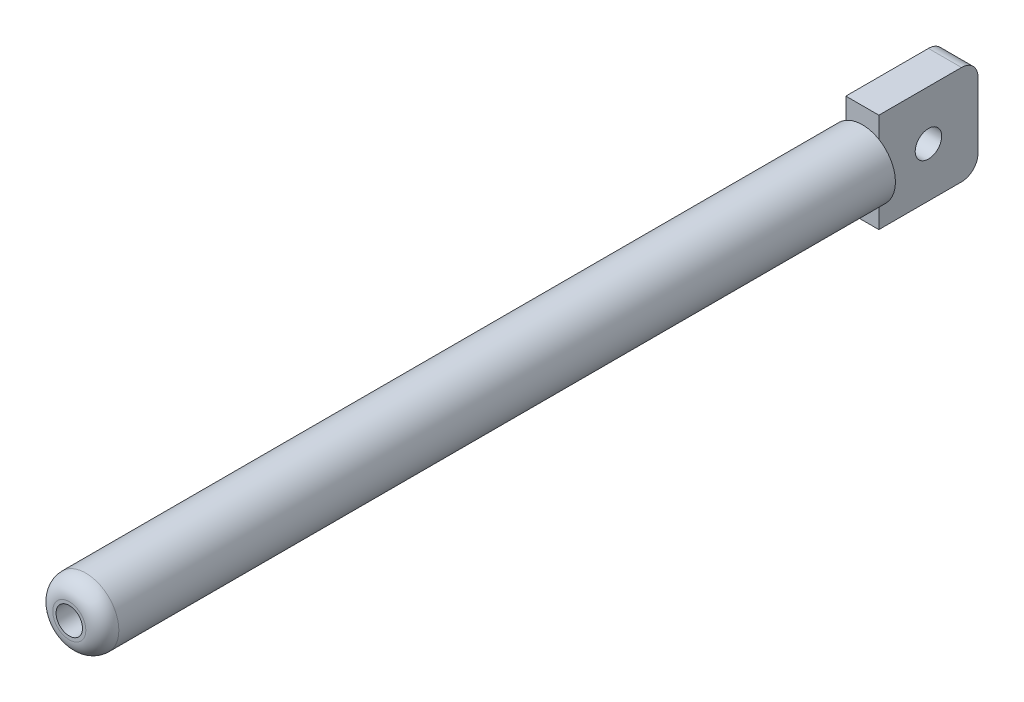
from build123d import *

# Parameters (mm, degrees)
SKETCH1_R           = 10
BOSS_EXTRUDE1_DEPTH = 240
SKETCH2_W           = 30
SKETCH2_H           = 30
BOSS_EXTRUDE2_DEPTH = 5
SKETCH3_R           = 4
CUT_EXTRUDE1_DEPTH  = 38
FILLET1_R           = 5
FILLET2_R           = 5
SKETCH4_R           = 4
CUT_EXTRUDE2_DEPTH  = 20


with BuildPart() as part:
    # Sketch1 → Boss-Extrude1 (new body)
    with BuildSketch(Plane.XY):
        Circle(SKETCH1_R)
    extrude(amount=BOSS_EXTRUDE1_DEPTH)

    # Sketch2 → Boss-Extrude2 (add, symmetric)
    with BuildSketch(Plane(origin=(0, 0, 0), x_dir=(0, 0, -1), z_dir=(1, 0, 0))):
        with Locations((15, 0)):
            Rectangle(SKETCH2_W, SKETCH2_H)
    extrude(amount=BOSS_EXTRUDE2_DEPTH, both=True)

    # Sketch3 → Cut-Extrude1 (cut)
    with BuildSketch(Plane(origin=(5, 0, 0), x_dir=(0, 0, -1), z_dir=(1, 0, 0))):
        with Locations((15, 0)):
            Circle(SKETCH3_R)
    extrude(amount=-CUT_EXTRUDE1_DEPTH, mode=Mode.SUBTRACT)

    # Fillet1
    fillet1_edges = [part.edges().sort_by_distance(p)[0] for p in [
        (0, -15, -30),
        (0, 15, -30),
    ]]
    fillet(fillet1_edges, radius=FILLET1_R)

    # Fillet2
    fillet2_edges = [part.edges().sort_by_distance(p)[0] for p in [
        (-10, 0, 240),
    ]]
    fillet(fillet2_edges, radius=FILLET2_R)

    # Sketch4 → Cut-Extrude2 (cut)
    with BuildSketch(Plane.XY.offset(240)):
        Circle(SKETCH4_R)
    extrude(amount=-CUT_EXTRUDE2_DEPTH, mode=Mode.SUBTRACT)


solid = part.part
